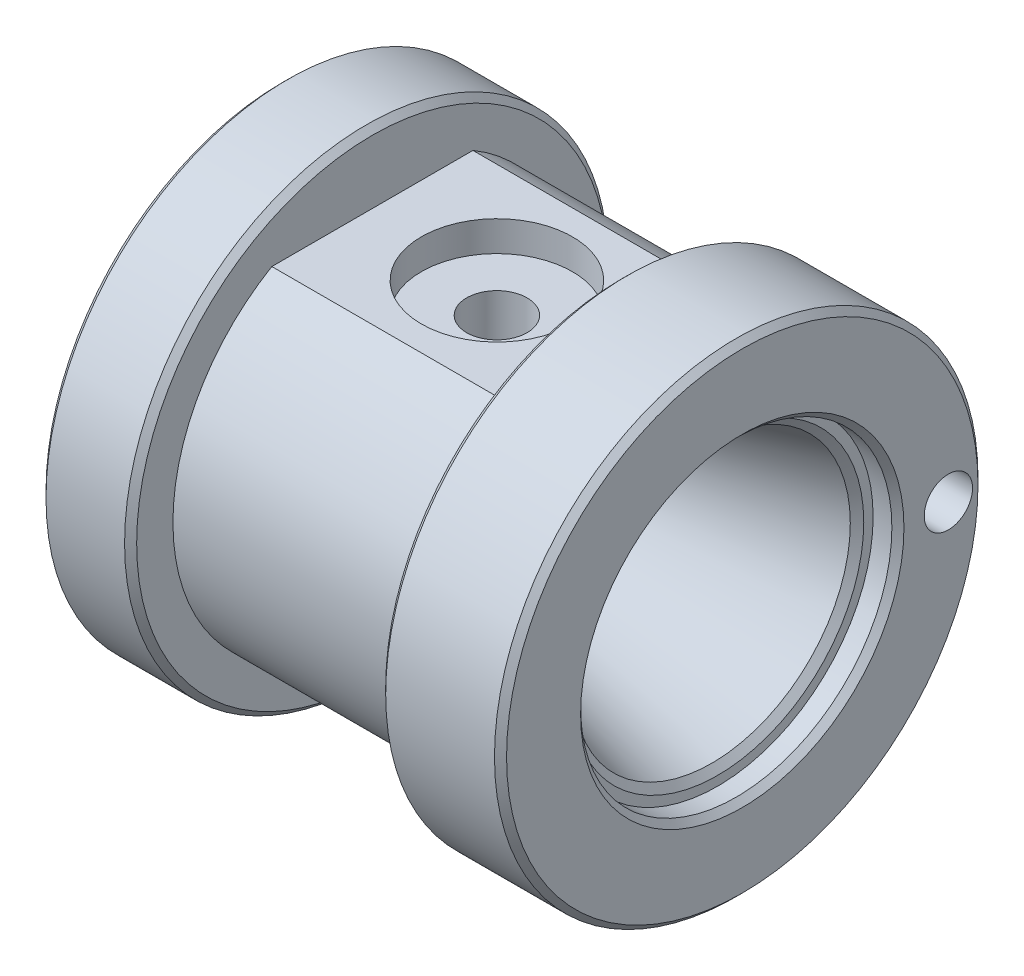
SolidWorks part; units mm, degrees
ref_plane "Front Plane" through (0, 0, 0) normal (0, 0, 1) x (1, 0, 0)
ref_plane "Top Plane" through (0, 0, 0) normal (0, 1, 0) x (1, 0, 0)
ref_plane "Right Plane" through (0, 0, 0) normal (1, 0, 0) x (0, 0, -1)
sketch "Sketch1" plane through (0, 0, 0) normal (0, 0, 1) x (1, 0, 0)
  line L0 (0, 26.75) -> (0, 40)
  line L1 (0, 40) -> (-20, 40)
  line L2 (-20, 40) -> (-20, 33)
  line L3 (-20, 33) -> (-61.2, 33)
  line L4 (-61.2, 33) -> (-61.2, 40)
  line L5 (-61.2, 40) -> (-76.2, 40)
  line L6 (-76.2, 40) -> (-76.2, 26)
  line L7 (-76.2, 26) -> (-75.2, 25)
  line L8 (-75.2, 25) -> (-65.7, 25)
  line L9 (-65.7, 25) -> (-65.7, 20.742)
  line L10 (23.5281, 0) -> (-116.1197, 0) construction
  line L11 (-52.2, 12) -> (-45.1, 12)
  line L12 (-44.1, 13) -> (-44.1, 14.65)
  line L13 (-44.1, 14.65) -> (-36, 14.65)
  line L14 (-36, 14.65) -> (-5.0659, 22.9388)
  line L15 (-4.1, 24.1976) -> (-4.1, 25.75)
  line L16 (-4.1, 25.75) -> (-1, 25.75)
  line L17 (-1, 25.75) -> (0, 26.75)
  line L18 (-5.0659, 22.9388) -> (-4.1, 24.1976)
  line L19 (-45.1, 12) -> (-44.1, 13)
  arc A0 (-65.7, 20.742) -> (-52.2, 12) centre (-68.9034, 1.0002) cw
  point P4 (-76.2, 25)
  point P13 (-4.1, 23.1976)
  point P14 (-44.1, 12)
  point P19 (0, 25.75)
  dimension "D4" = 20
  dimension "D2" = 15
  dimension "D3" = 20
  dimension "D7" = 10.5
  dimension "D8" = 24
  dimension "D9" = 40
  dimension "D10" = 36
  dimension "D11" = 4.1
revolve "Revolve1" add sketch "Sketch1" angle 360 about L10
chamfer "Chamfer1" distance 1 angle 45 4 edges at (0, 0, -40) (-20, 0, -40) (-76.2, 0, -40) (-61.2, 0, -40)
sketch "Sketch2" plane through (0, 0, 0) normal (0, 0, 1) x (1, 0, 0)
  line L0 (-61.2, 28.5) -> (-61.2, 56.2708)
  line L3 (-20, 28.5) -> (-61.2, 28.5)
  line L4 (-20, -28.5) -> (-61.2, -28.5)
  line L5 (-61.2, 56.2708) -> (-20, 56.2708)
  line L6 (-20, 56.2708) -> (-20, 28.5)
  line L7 (-61.2, -28.5) -> (-61.2, -59.3239)
  line L8 (-61.2, -59.3239) -> (-20, -59.3239)
  line L9 (-20, -59.3239) -> (-20, -28.5)
extrude "Cut-Extrude1" cut sketch "Sketch2" against normal through all and the other way through all
sketch "Sketch3" plane through (0, 28.5, 0) normal (0, 1, 0) x (1, 0, 0)
  circle A0 centre (-40.6, 0) radius 12.5
  dimension "D1" = 25
extrude "Cut-Extrude2" cut sketch "Sketch3" against normal blind 5
sketch "Sketch4" plane through (0, 23.5, 0) normal (0, 1, 0) x (1, 0, 0)
  circle A0 centre (-40.6, 0) radius 5
  dimension "D1" = 10
extrude "Cut-Extrude3" cut sketch "Sketch4" against normal blind 19
mirror "Mirror1" about plane through (0, 0, 0) normal (0, 1, 0) of "Cut-Extrude2", "Cut-Extrude3"
sketch "Sketch5" plane through (-76.2, 0, 0) normal (-1, 0, 0) x (0, 0, 1)
  circle A1 centre (-34.0977, 0) radius 4
  dimension "D1" = 8
extrude "Cut-Extrude4" cut sketch "Sketch5" against normal blind 10
sketch "Sketch6" plane through (0, 0, 0) normal (1, 0, 0) x (0, 0, -1)
  circle A1 centre (34.1, 0) radius 4
  dimension "D2" = 8
extrude "Cut-Extrude5" cut sketch "Sketch6" against normal blind 13
